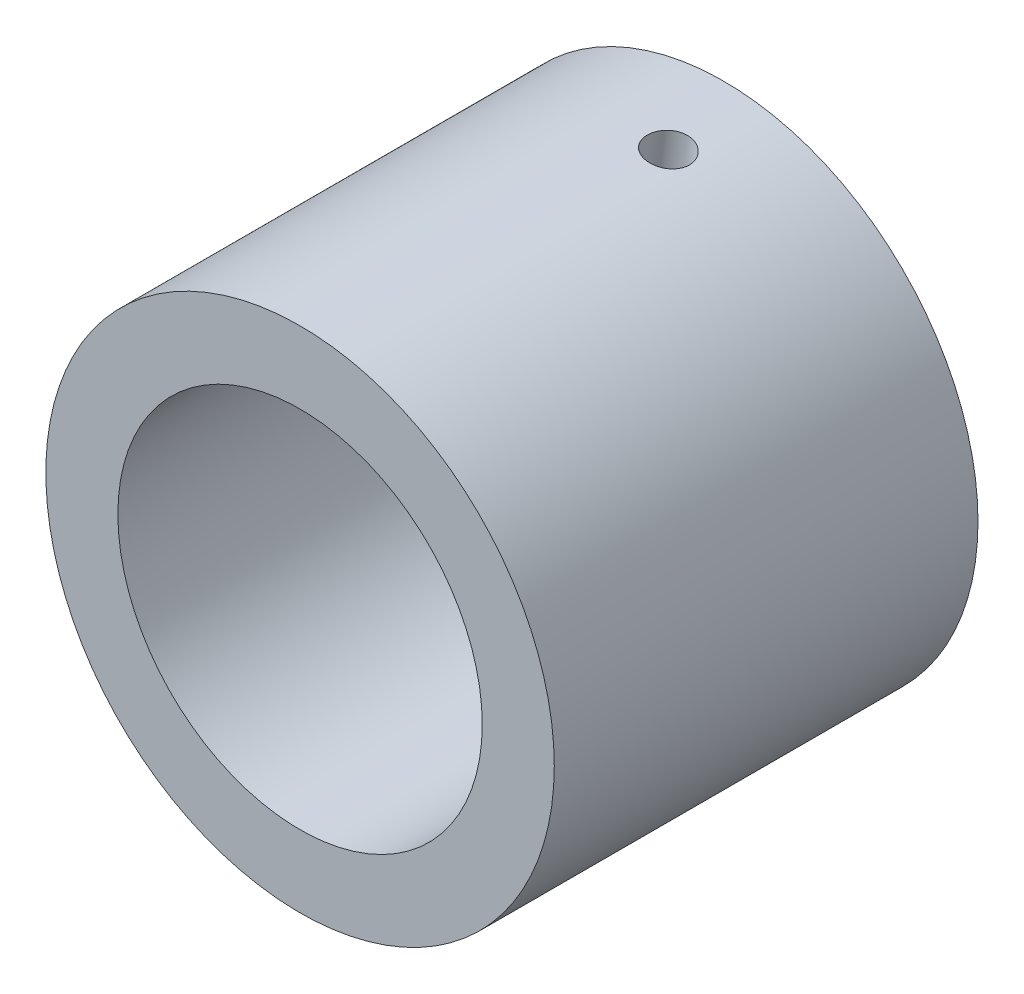
from build123d import *

# Parameters (mm, degrees)
SKETCH1_R             = 30
SKETCH1_R_2           = 21.5
BOSS_EXTRUDE1_DEPTH   = 50
M6_TAPPED_HOLE1_D     = 5
M6_TAPPED_HOLE1_DEPTH = 18
M6_TAPPED_HOLE1_TIP   = 1.502151548
BOSS_EXTRUDE2_START   = 24
SKETCH4_R             = 25
SKETCH4_R_2           = 21.5
BOSS_EXTRUDE2_DEPTH   = 24
SKETCH6_R             = 25
SKETCH6_R_2           = 21.5
CUT_EXTRUDE1_DEPTH    = 24


with BuildPart() as part:
    # Sketch1 → Boss-Extrude1 (new body)
    with BuildSketch(Plane.XY):
        Circle(SKETCH1_R)
        Circle(SKETCH1_R_2, mode=Mode.SUBTRACT)
    extrude(amount=-BOSS_EXTRUDE1_DEPTH)

    # M6 Tapped Hole1
    with Locations(Plane(origin=(3.471069712, 29.798518001, -40), x_dir=(0.993283933364, -0.115702323745, 0), z_dir=(0.115702323745, 0.993283933364, 0))):
        with Locations((0, 0)):
            Hole(M6_TAPPED_HOLE1_D / 2, depth=M6_TAPPED_HOLE1_DEPTH)
            with Locations((0, 0, -(M6_TAPPED_HOLE1_DEPTH + M6_TAPPED_HOLE1_TIP / 2))):  # 118° drill point
                Cone(0, M6_TAPPED_HOLE1_D / 2, M6_TAPPED_HOLE1_TIP, mode=Mode.SUBTRACT)

    # Sketch4 → Boss-Extrude2 (add)
    with BuildSketch(Plane.XY.offset(BOSS_EXTRUDE2_START)):
        Circle(SKETCH4_R)
        Circle(SKETCH4_R_2, mode=Mode.SUBTRACT)
    extrude(amount=-BOSS_EXTRUDE2_DEPTH)

    # Sketch6 → Cut-Extrude1 (cut)
    with BuildSketch(Plane.XY.offset(24)):
        Circle(SKETCH6_R)
        Circle(SKETCH6_R_2, mode=Mode.SUBTRACT)
    extrude(amount=-CUT_EXTRUDE1_DEPTH, mode=Mode.SUBTRACT)


solid = part.part
